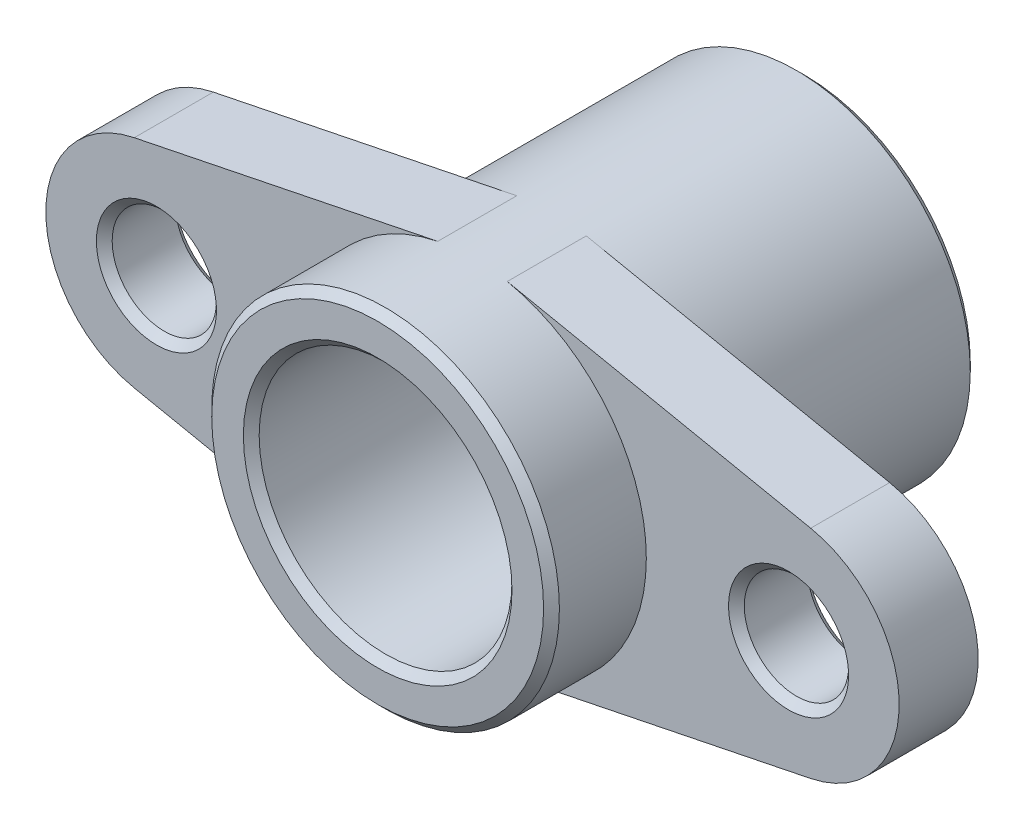
SolidWorks part; units mm, degrees
material "45(Ni)"
ref_plane "Front Plane" through (0, 0, 0) normal (0, 0, 1) x (1, 0, 0)
ref_plane "Top Plane" through (0, 0, 0) normal (0, 1, 0) x (1, 0, 0)
ref_plane "Right Plane" through (0, 0, 0) normal (1, 0, 0) x (0, 0, -1)
sketch "Sketch1" plane through (0, 0, 0) normal (0, 0, 1) x (1, 0, 0)
  circle A0 centre (0, 0) radius 8
  circle A1 centre (0, 0) radius 11
  dimension "D1" = 16
  dimension "D2" = 3
extrude "Boss-Extrude1" add sketch "Sketch1" along normal blind 30
sketch "Sketch2" plane through (0, 0, 30) normal (0, 0, 1) x (1, 0, 0)
  line L0 (-21.4, 6.8586) -> (-2.2, 10.7778)
  line L1 (-20, 0) -> (0, 0) construction
  line L2 (0, 0) -> (20, 0) construction
  line L3 (2.2, 10.7778) -> (21.4, 6.8586)
  line L4 (-21.4, -6.8586) -> (-2.2, -10.7778)
  line L5 (2.2, -10.7778) -> (21.4, -6.8586)
  arc A0 (-21.4, 6.8586) -> (-21.4, -6.8586) centre (-20, 0) ccw
  arc A1 (21.4, -6.8586) -> (21.4, 6.8586) centre (20, 0) ccw
  circle A2 centre (0, 0) radius 11 construction
  arc A3 (-2.2, -10.7778) -> (2.2, -10.7778) centre (0, 0) ccw
  arc A4 (2.2, 10.7778) -> (-2.2, 10.7778) centre (0, 0) ccw
  circle A5 centre (0, 0) radius 8 construction
  circle A6 centre (0, 0) radius 8
  dimension "D2" = 14
  dimension "D1" = 20
extrude "Boss-Extrude2" add sketch "Sketch2" against normal blind 14
hole_wizard "Hole size per socket head cap screw type1" positions "3DSketch1" profile "Sketch3" counterbore size "M8" standard "Gb" end condition through all
sketch3d "3DSketch1"
  arc A0 (-21.4, 6.8586, 30) -> (-21.4, -6.8586, 30) centre (-20, 0, 30) ccw construction
  arc A1 (21.4, -6.8586, 30) -> (21.4, 6.8586, 30) centre (20, 0, 30) ccw construction
  point P0 (-20, 0, 30)
  point P2 (20, 0, 30)
  point P9 (-20, 0, 37)
  point P14 (20, 0, 37)
sketch "Sketch3" plane through (-20, 0, 30) normal (1, 0, 0) x (0, -1, 0)
  line L0 (0, 0) -> (0, 30)
  line L1 (0, 30) -> (3.3, 30)
  line L3 (3.3, 30) -> (3.3, 9)
  line L4 (3.3, 9) -> (7.5, 9)
  line L5 (7.5, 9) -> (7.5, 0)
  line L7 (7.5, 0) -> (0, 0)
  line L11 (0, -6.35) -> (0, 107.95) construction
  dimension "通孔孔直径" = 6.6
  dimension "通孔孔深度" = 30
  dimension "柱形沉头孔直径" = 15
  dimension "柱形沉头孔深度" = 9
sketch "Sketch5" plane through (0, 0, 30) normal (0, 0, 1) x (1, 0, 0)
  circle A0 centre (0, 0) radius 11
  arc A1 (2.2, 10.7778) -> (-2.2, 10.7778) centre (0, 0) ccw construction
extrude "Cut-Extrude2" cut sketch "Sketch5" against normal up to surface (9 mm away) flip side to cut up to face at (-19.9155, 0, 21)
sketch "Sketch6" plane through (0, 0, 30) normal (0, 0, 1) x (1, 0, 0)
  circle A0 centre (0, 0) radius 11 construction
  circle A1 centre (0, 0) radius 11
extrude "Cut-Extrude3" cut sketch "Sketch6" against normal blind 3
chamfer "Chamfer1" distance 0.5 angle 45 8 edges at (11, 0, 27) (8, 0, 27) (11, 0, 0) (23.3, 0, 16) (23.3, 0, 21) (8, 0, 0) (-16.7, 0, 16) (-16.7, 0, 21)
